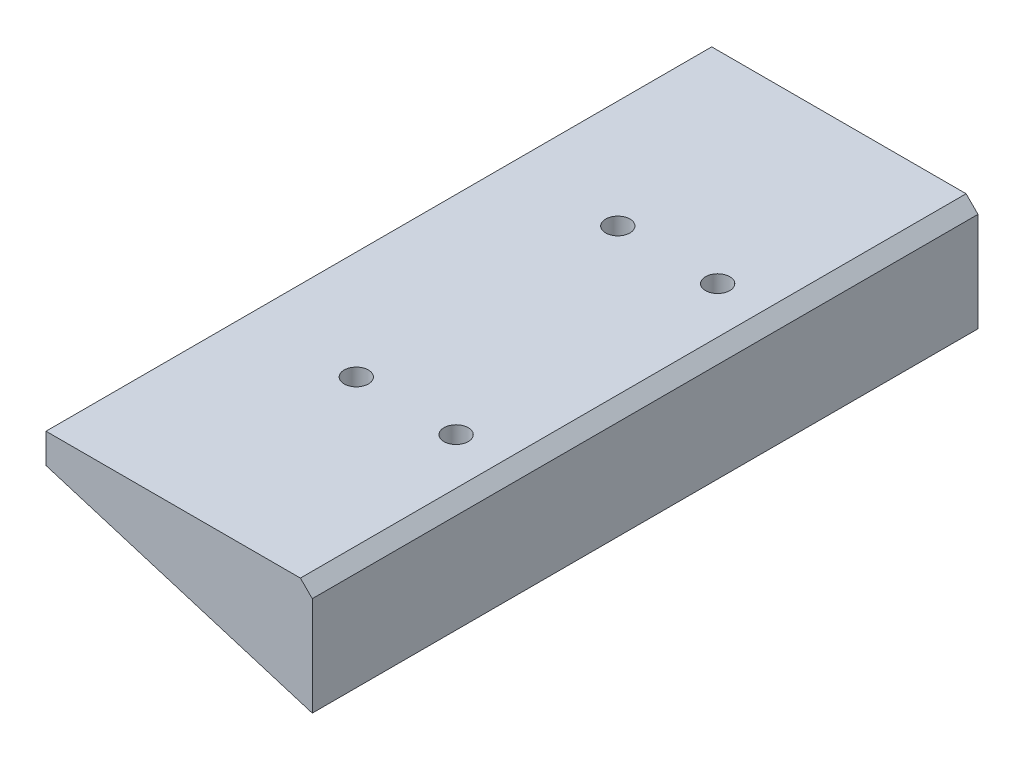
from build123d import *

# Parameters (mm, degrees)
BOSS_EXTRUDE1_DEPTH = 280
M12_TAPPED_HOLE1_D  = 10.2


with BuildPart() as part:
    # Sketch1 → Boss-Extrude1 (new body)
    with BuildSketch(Plane.XY):
        Polygon((0, 0), (0, 12.5), (107, 12.5), (112, 7.5), (112, -34.2), align=None)
    extrude(amount=BOSS_EXTRUDE1_DEPTH)

    # M12 Tapped Hole1 (through all)
    with Locations(Plane(origin=(0, 12.5, 0), x_dir=(-1, 0, 0), z_dir=(0, 1, 0))):
        with Locations((-45.5, 195), (-45.5, 85), (-87.5, 85), (-87.5, 195)):
            Hole(M12_TAPPED_HOLE1_D / 2)


solid = part.part
